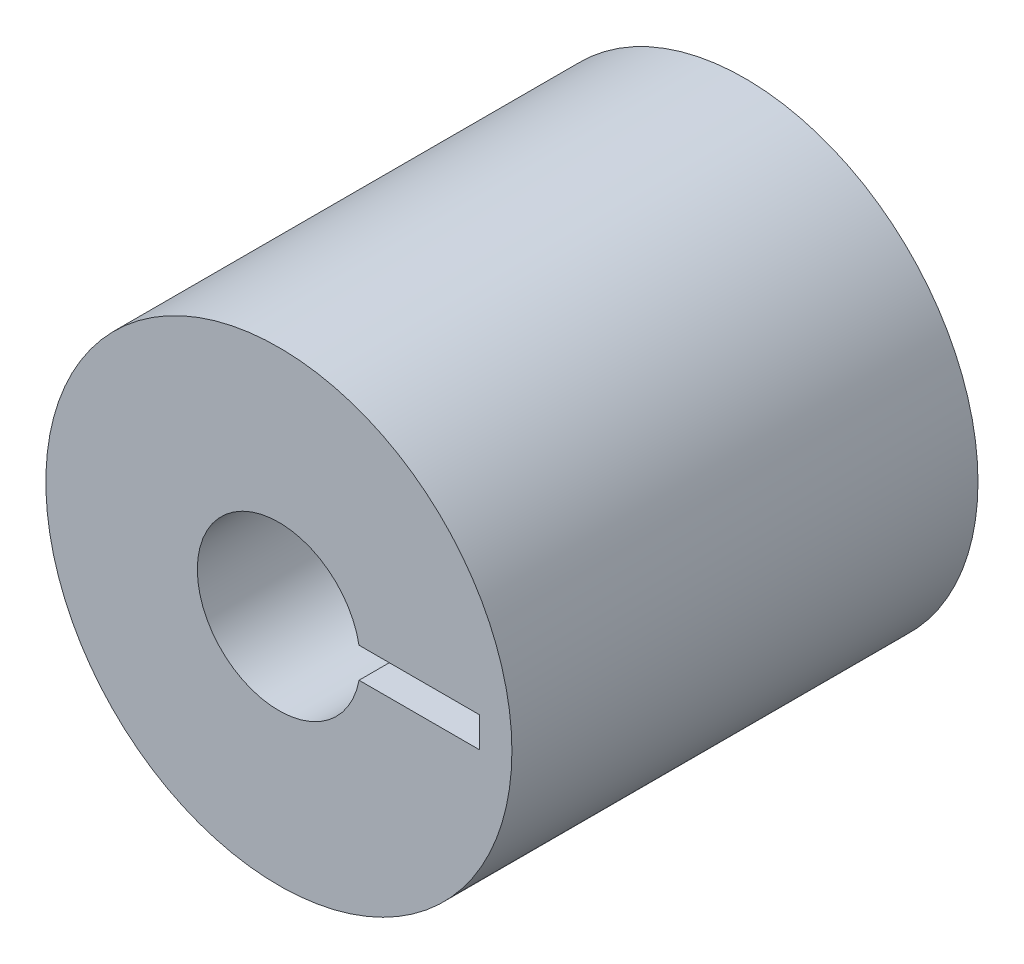
from build123d import *

# Parameters (mm, degrees)
SKETCH_1_R          = 20
EXTRUDE_1_DEPTH     = 40
SKETCH_2_R          = 4
CUT_EXTRUDE_1_DEPTH = 49.989794856
SKETCH_3_R          = 7
CUT_EXTRUDE_2_DEPTH = 28
CUT_EXTRUDE_3_DEPTH = 13
CUT_EXTRUDE_START   = -13
CUT_EXTRUDE_4_DEPTH = 13


with BuildPart() as part:
    # 草图1 → 凸台-拉伸1 (new body)
    with BuildSketch(Plane.XY):
        Circle(SKETCH_1_R)
    extrude(amount=EXTRUDE_1_DEPTH)

    # 草图2 → 切除-拉伸1 (cut, through all)
    with BuildSketch(Plane.XY.offset(40)):
        Circle(SKETCH_2_R)
    extrude(amount=-CUT_EXTRUDE_1_DEPTH, mode=Mode.SUBTRACT)

    # 草图3 → 切除-拉伸2 (cut)
    with BuildSketch(Plane.XY.offset(40)):
        Circle(SKETCH_3_R)
    extrude(amount=-CUT_EXTRUDE_2_DEPTH, mode=Mode.SUBTRACT)

    # 草图4 → 切除-拉伸3 (cut)
    with BuildSketch(Plane.XY.offset(40)):
        with BuildLine():
            Line((17.228226516, -1.3), (17.228226516, 1.3))
            Line((17.228226516, 1.3), (6.878226516, 1.3))
            ThreePointArc((6.878226516, 1.3), (7, 0), (6.878226516, -1.3))
            Line((6.878226516, -1.3), (17.228226516, -1.3))
        make_face()
    extrude(amount=-CUT_EXTRUDE_3_DEPTH, mode=Mode.SUBTRACT)

    # 草图5 → 切除-拉伸4 (cut)
    with BuildSketch(Plane(origin=(0, 0, 0), x_dir=(-1, 0, 0), z_dir=(0, 0, -1)).offset(CUT_EXTRUDE_START)):
        with BuildLine():
            Line((16.948468057, -0.64), (16.948468057, 0.64))
            Line((16.948468057, 0.64), (3.948468057, 0.64))
            ThreePointArc((3.948468057, 0.64), (4, 0), (3.948468057, -0.64))
            Line((3.948468057, -0.64), (16.948468057, -0.64))
        make_face()
    extrude(amount=CUT_EXTRUDE_4_DEPTH, mode=Mode.SUBTRACT)


solid = part.part
